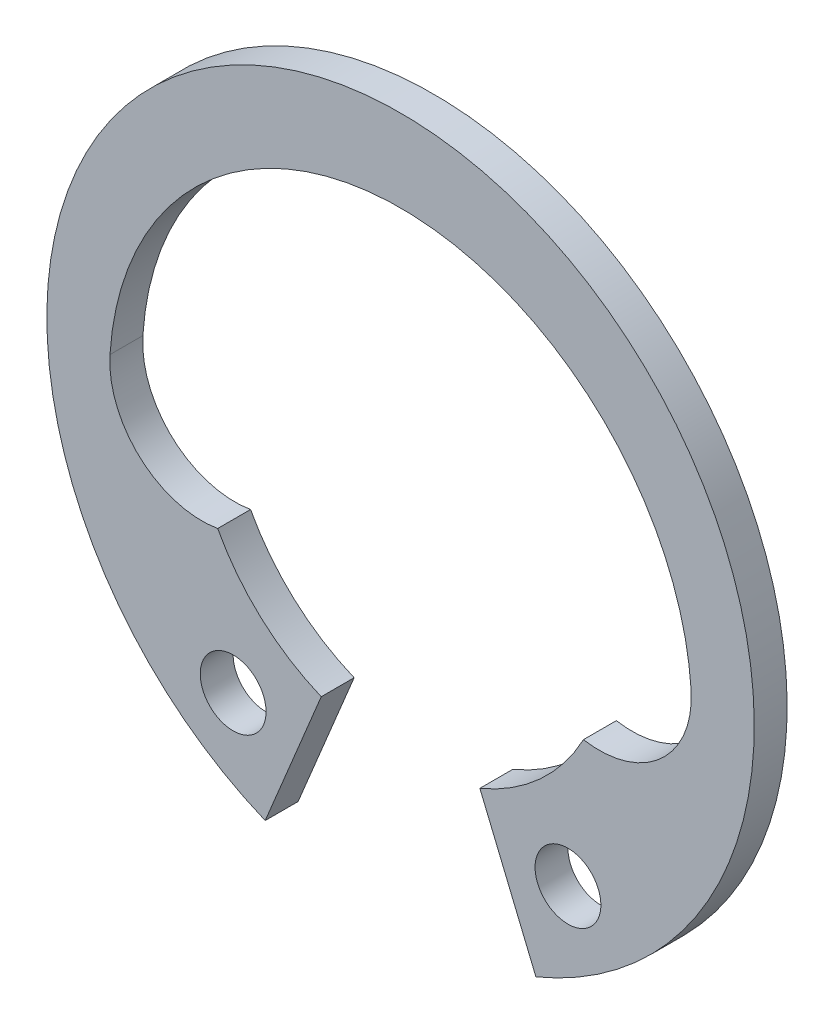
SolidWorks part; units mm, degrees
ref_plane "Front" through (0, 0, 0) normal (0, 0, 1) x (1, 0, 0)
ref_plane "Top" through (0, 0, 0) normal (0, 1, 0) x (1, 0, 0)
ref_plane "Right" through (0, 0, 0) normal (1, 0, 0) x (0, 0, -1)
sketch "Sketch1" plane through (0, 0, 0) normal (0, 0, 1) x (1, 0, 0)
  line L0 (-2.4109, -5.8204) -> (-4.1138, -9.9317)
  line L1 (2.4109, -5.8204) -> (4.1138, -9.9317)
  line L2 (0, 17.9027) -> (0, -23.5886) construction
  arc A0 (4.1138, -9.9317) -> (-4.1138, -9.9317) centre (0, 0) ccw
  arc A1 (8.8313, -0.0256) -> (-8.8313, -0.0256) centre (0, -0.6) ccw
  arc A2 (3.3293, -8.0378) -> (-3.3293, -8.0378) centre (0, 0) ccw construction
  circle A3 centre (5.0879, -7.0571) radius 1
  arc A4 (-8.8313, -0.0256) -> (-5.5581, -2.966) centre (-6.0372, -0.2073) ccw
  arc A5 (-5.5581, -2.966) -> (-2.4109, -5.8204) centre (0, 0) ccw
  circle A6 centre (-5.0879, -7.0571) radius 1
  arc A8 (5.5581, -2.966) -> (2.4109, -5.8204) centre (0, 0) cw
  arc A9 (8.8313, -0.0256) -> (5.5581, -2.966) centre (6.0372, -0.2073) cw
  dimension "R2" = 2.8
  dimension "d1" = 2
  dimension "d0" = 17.7
  dimension "D" = 21.5
  dimension "R" = 8.7
  dimension "a" = 4.45
  dimension "c" = 0.6
  dimension "Angle" = 45
  dimension "B" = 4
  dimension "B1" = 2
extrude "Body" add sketch "Sketch1" against normal blind 1
